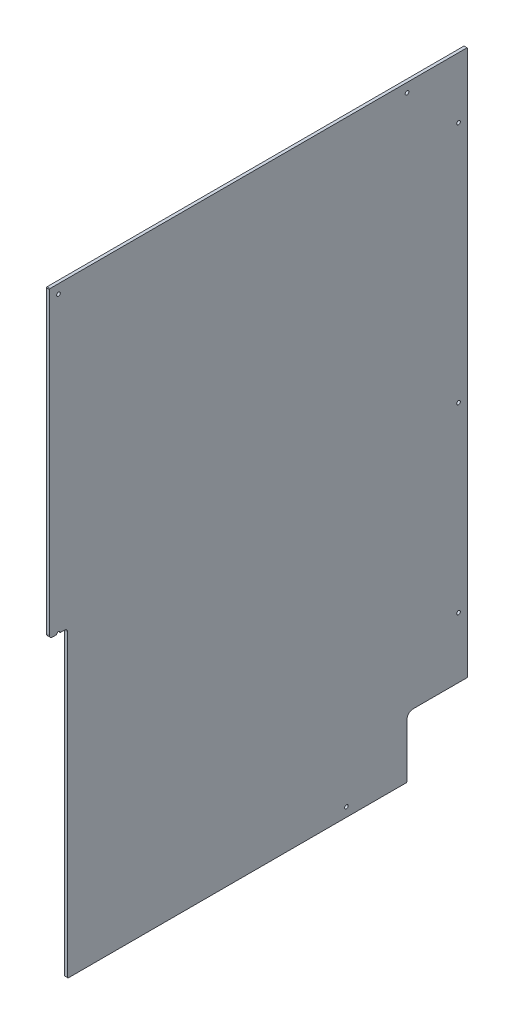
SolidWorks part; units mm, degrees
material "PC(透明)"
ref_plane "前基準面" through (0, 0, 0) normal (0, 0, 1) x (1, 0, 0)
ref_plane "上基準面" through (0, 0, 0) normal (0, 1, 0) x (1, 0, 0)
ref_plane "右基準面" through (0, 0, 0) normal (1, 0, 0) x (0, 0, -1)
sketch "草图1" plane through (0, 0, 0) normal (1, 0, 0) x (0, 0, -1)
  line L1 (345, 500) -> (-345, 500)
  line L2 (345, 500) -> (345, -500)
  line L3 (345, -500) -> (-345, -500)
  line L4 (-345, 500) -> (-345, -500)
  line L5 (345, 500) -> (-345, -500) construction
  line L6 (345, -500) -> (-345, 500) construction
  point P0 (0, 0)
  dimension "D1" = 690
  dimension "D2" = 1000
extrude "凸台-拉伸1" add sketch "草图1" along normal blind 5
chamfer "倒角1" distance 1 angle 45 4 edges at (2.5, -500, -345) (2.5, -500, 345) (2.5, 500, -345) (2.5, 500, 345)
sketch "草图2" plane through (0, 0, 0) normal (-1, 0, 0) x (0, 0, 1)
  line L0 (-345, -499) -> (-345, 499) construction
  line L1 (-344, 500) -> (344, 500) construction
  line L2 (58.8862, 0) -> (0, 0) construction
  line L3 (0, 0) -> (0, 69.8386) construction
  line L5 (330, -485) -> (-330, -485) construction
  line L6 (330, -485) -> (330, 485) construction
  line L7 (330, 485) -> (-330, 485) construction
  line L8 (-330, -485) -> (-330, 485) construction
  line L9 (330, -485) -> (-330, 485) construction
  line L10 (330, 485) -> (-330, -485) construction
  circle A0 centre (-330, 485) radius 3 construction
  circle A1 centre (-330, -485) radius 3
  circle A2 centre (330, -485) radius 3
  circle A3 centre (330, 485) radius 3
  circle A8 centre (330, 0) radius 3
  circle A9 centre (-330, 0) radius 3
  dimension "D1" = 6
  dimension "D2" = 15
  dimension "D3" = 15
extrude "切除-拉伸1" cut sketch "草图2" against normal through all
sketch "草图3" plane through (0, 0, 0) normal (-1, 0, 0) x (0, 0, 1)
  line L0 (344, -500) -> (-344, -500) construction
  line L1 (-245, -500) -> (-345, -500)
  line L2 (-245, -500) -> (-245, -400)
  line L3 (-245, -400) -> (-345, -400)
  line L4 (-345, -500) -> (-345, -400)
  line L5 (-345, -499) -> (-345, 499) construction
  line L6 (0, 0) -> (-710, 0) construction
  line L7 (-345, 500) -> (-345, 400) construction
  line L8 (-245, 400) -> (-345, 400) construction
  line L9 (-245, 500) -> (-245, 400) construction
  line L10 (-245, 500) -> (-345, 500) construction
  dimension "D1" = 100
  dimension "D2" = 100
extrude "切除-拉伸2" cut sketch "草图3" against normal through all
hole_wizard "Ø6.0 (6) 直径孔1" positions "草图5" profile "草图4" hole size "Ø6.0" standard "GB"
sketch "草图5" plane through (0, -600, 465) normal (-1, 0, 0) x (0, 0, 1)
  line L0 (-809, 1100) -> (-121, 1100) construction
  line L1 (-810, 200) -> (-810, 1099) construction
  line L4 (-710, 200) -> (-810, 200) construction
  line L5 (-710, 100) -> (-710, 200) construction
  line L6 (-121, 100) -> (-710, 100) construction
  line L8 (-810, 200) -> (-810, 1099) construction
  line L9 (-809, 1100) -> (-121, 1100) construction
  point P1 (-710, 1085)
  point P3 (-795, 1000)
  point P5 (-795, 300)
  point P7 (-610, 115)
  dimension "D1" = 15
  dimension "D2" = 15
  dimension "D3" = 100
  dimension "D4" = 100
  dimension "D5" = 100
  dimension "D6" = 100
  dimension "D7" = 15
  dimension "D8" = 15
sketch "草图4" plane through (0, 485, -245) normal (0, 1, 0) x (0, 0, 1)
  line L0 (0, 0) -> (0, 8)
  line L1 (0, 8) -> (3, 5)
  line L2 (3, 5) -> (3, 0)
  line L5 (3, 0) -> (0, 0)
  line L10 (0, 8) -> (-3, 5) construction
  line L11 (0, -6.35) -> (0, 107.95) construction
  dimension "孔直径" = 6
  dimension "孔深度" = 5
  dimension "导头角度" = 90
fillet "圆角1" radius 10 1 edges at (2.5, -400, -245)
sketch "草图6" plane through (0, 0, 0) normal (-1, 0, 0) x (0, 0, 1)
  line L1 (345, -500) -> (315, -500)
  line L2 (345, -500) -> (345, 0)
  line L3 (345, 0) -> (315, 0)
  line L4 (315, -500) -> (315, 0)
  line L5 (345, 499) -> (345, -499) construction
  line L6 (344, -500) -> (-245, -500) construction
  dimension "D1" = 30
  dimension "D2" = 500
extrude "切除-拉伸3" cut sketch "草图6" against normal blind 10
chamfer "倒角2" distance 1 angle 45 3 edges at (2.5, -400, -345) (2.5, -500, -245) (2.5, -500, 315)
fillet "圆角2" radius 5 2 edges at (2.5, 0, 345) (2.5, 0, 315)
